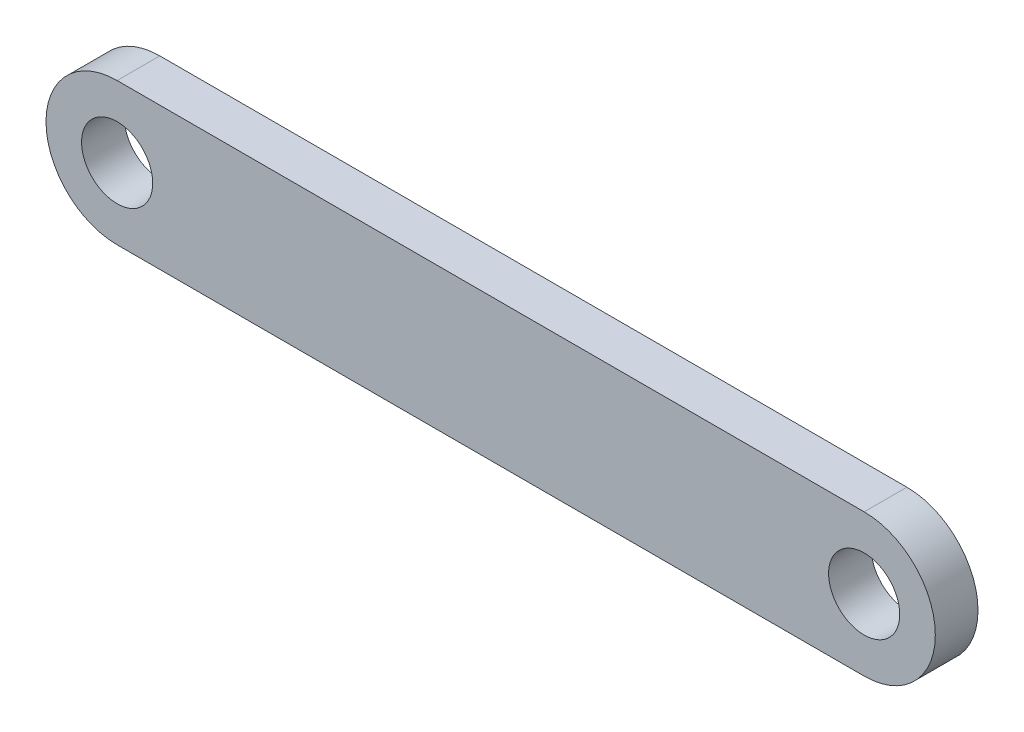
SolidWorks part; units mm, degrees
material "AISI 304"
ref_plane "Front Plane" through (0, 0, 0) normal (0, 0, 1) x (1, 0, 0)
ref_plane "Top Plane" through (0, 0, 0) normal (0, 1, 0) x (1, 0, 0)
ref_plane "Right Plane" through (0, 0, 0) normal (1, 0, 0) x (0, 0, -1)
other "Configuration Table"
sketch "Sketch1" plane through (0, 0, 0) normal (0, 0, 1) x (1, 0, 0)
  line L0 (0, 0) -> (105, 0) construction
  line L1 (0, 10) -> (105, 10)
  line L2 (0, -10) -> (105, -10)
  arc A0 (0, 10) -> (0, -10) centre (0, 0) ccw
  arc A1 (105, -10) -> (105, 10) centre (105, 0) ccw
  circle A2 centre (0, 0) radius 5
  circle A3 centre (105, 0) radius 5
  point P3 (52.5, 0)
  dimension "D2" = 10
  dimension "D3" = 10
  dimension "D4" = 10
  dimension "D1" = 105
extrude "Boss-Extrude1" add sketch "Sketch1" along normal mid plane 6
